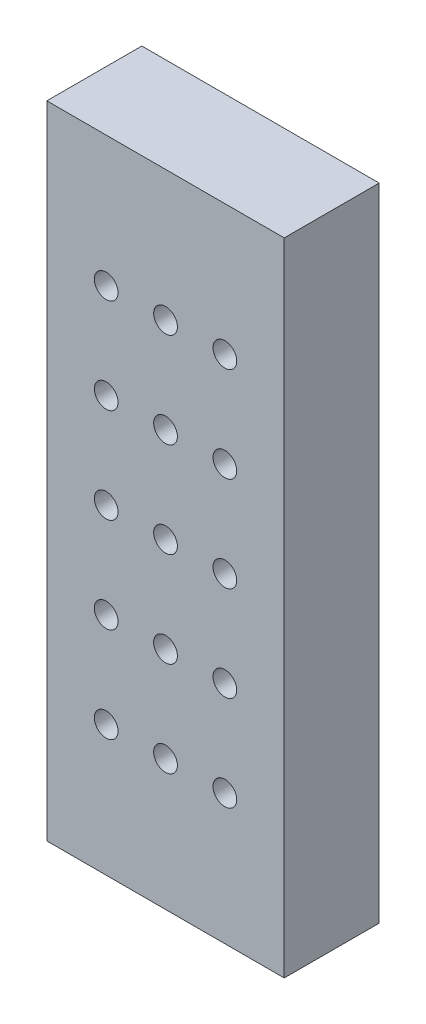
SolidWorks part; units mm, degrees
ref_plane "前视基准面" through (0, 0, 0) normal (0, 0, 1) x (1, 0, 0)
ref_plane "上视基准面" through (0, 0, 0) normal (0, 1, 0) x (1, 0, 0)
ref_plane "右视基准面" through (0, 0, 0) normal (1, 0, 0) x (0, 0, -1)
sketch "草图1" plane through (0, 0, 0) normal (0, 0, 1) x (1, 0, 0)
  line L1 (-5, -13.5) -> (5, -13.5)
  line L2 (-5, -13.5) -> (-5, 13.5)
  line L3 (-5, 13.5) -> (5, 13.5)
  line L4 (5, -13.5) -> (5, 13.5)
  line L5 (-5, -13.5) -> (5, 13.5) construction
  line L6 (-5, 13.5) -> (5, -13.5) construction
  point P0 (0, 0)
  dimension "D1" = 10
  dimension "D2" = 27
extrude "凸台-拉伸1" add sketch "草图1" along normal blind 4
sketch "草图2" plane through (0, 0, 4) normal (0, 0, 1) x (1, 0, 0)
  circle A0 centre (0, 0) radius 0.5
  circle A1 centre (-2.5, 0) radius 0.5
  circle A2 centre (2.5, 0) radius 0.5
extrude "切除-拉伸1" cut sketch "草图2" against normal up to next
pattern_linear "阵列(线性)2" count 3 spacing 4 along (0, -1, 0) of "切除-拉伸1"
mirror "镜向1" about plane through (0, 0, 0) normal (0, 1, 0) of "阵列(线性)2"
sketch "草图3" plane through (0, 0, 0) normal (0, 0, -1) x (-1, 0, 0)
  line L0 (5, 13.5) -> (5, -13.5) construction
  line L1 (-1.8, 12.3) -> (1.8, 12.3)
  line L2 (-3.8, 10.3) -> (-3.8, -10.3)
  line L3 (-1.8, -12.3) -> (1.8, -12.3)
  line L4 (3.8, 10.3) -> (3.8, -10.3)
  line L5 (-3.8, 12.3) -> (3.8, -12.3) construction
  line L6 (-3.8, -12.3) -> (3.8, 12.3) construction
  line L7 (-5, 13.5) -> (5, 13.5) construction
  arc A0 (-3.8, -10.3) -> (-1.8, -12.3) centre (-1.8, -10.3) ccw
  arc A1 (1.8, -12.3) -> (3.8, -10.3) centre (1.8, -10.3) ccw
  arc A2 (-1.8, 12.3) -> (-3.8, 10.3) centre (-1.8, 10.3) ccw
  arc A3 (1.8, 12.3) -> (3.8, 10.3) centre (1.8, 10.3) cw
  point P0 (0, 0)
equation "\"D3@草图2\"=\"D2@草图2\""
equation "\"D3@草图3\"=\"D2@草图3\""
